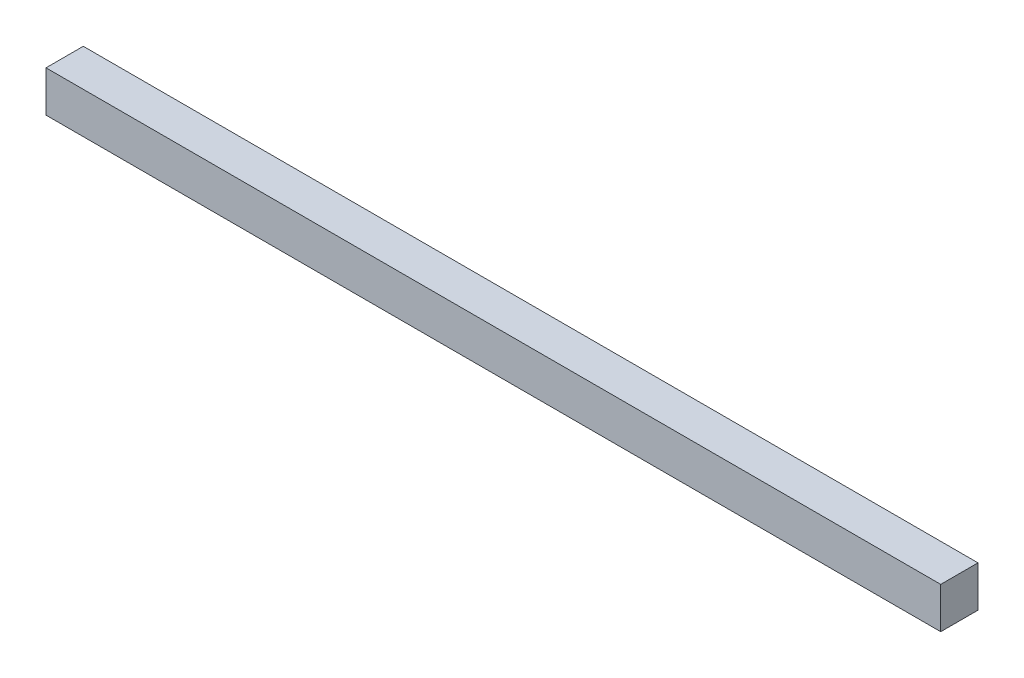
from build123d import *

# Parameters (mm, degrees)
SKETCH1_W           = 480
SKETCH1_H           = 22
BOSS_EXTRUDE1_DEPTH = 20


with BuildPart() as part:
    # Sketch1 → Boss-Extrude1 (new body)
    with BuildSketch(Plane.XY):
        with Locations((240, 11)):
            Rectangle(SKETCH1_W, SKETCH1_H)
    extrude(amount=BOSS_EXTRUDE1_DEPTH)


solid = part.part
